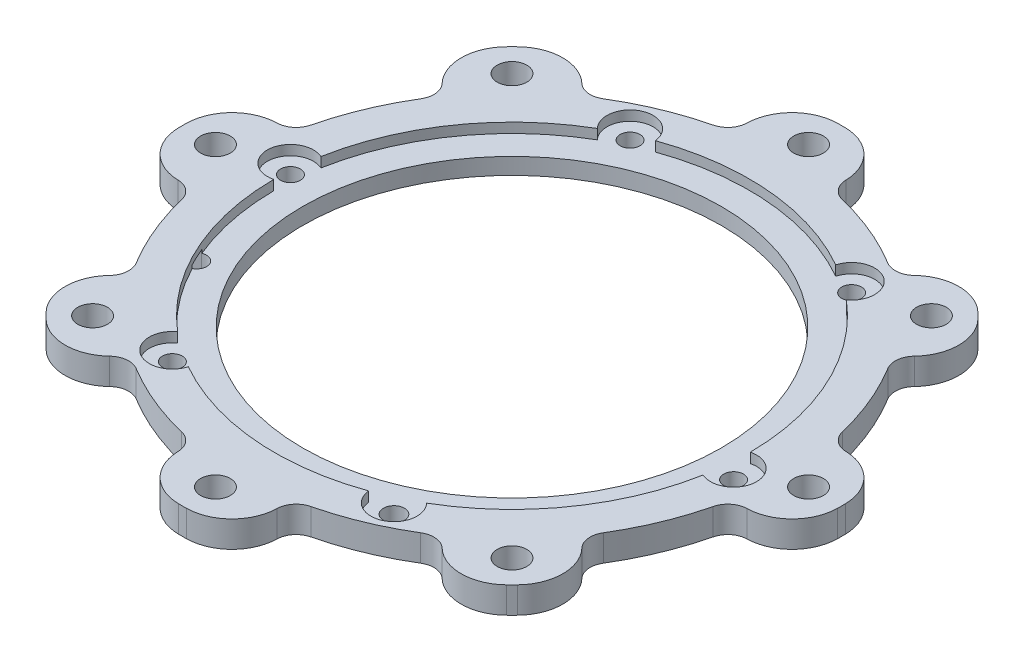
from build123d import *

# Parameters (mm, degrees)
SKETCH1_R           = 50
SKETCH1_R_2         = 30
BOSS_EXTRUDE1_DEPTH = 4
SKETCH2_R           = 39
SKETCH2_R_2         = 30
BOSS_EXTRUDE2_DEPTH = 1
SKETCH3_R           = 31.75
CUT_EXTRUDE1_DEPTH  = 1
SKETCH4_R           = 2.25
CUT_EXTRUDE2_DEPTH  = 10
CIRPATTERN1_COUNT   = 8
SKETCH5_R           = 31.75
CUT_EXTRUDE3_DEPTH  = 27
SKETCH6_R           = 3.5
CUT_EXTRUDE4_DEPTH  = 2.5
CIRPATTERN2_COUNT   = 6
SKETCH7_R           = 1.5
SKETCH7_R_2         = 1.597835056
CUT_EXTRUDE5_DEPTH  = 15
CUT_EXTRUDE6_DEPTH  = 13
CIRPATTERN3_COUNT   = 8
FILLET1_R           = 3
SKETCH9_R           = 36
CUT_EXTRUDE7_DEPTH  = 2.5
FILLET2_R           = 7
CUT_EXTRUDE8_START  = -1
SKETCH10_R          = 50
CUT_EXTRUDE8_DEPTH  = 1
SKETCH12_R          = 1.5
CUT_EXTRUDE9_DEPTH  = 3
CUT_EXTRUDE10_REACH = 72.824


with BuildPart() as part:
    # Sketch1 → Boss-Extrude1 (new body)
    with BuildSketch(Plane(origin=(0, 0, 0), x_dir=(1, 0, 0), z_dir=(0, 1, 0))):
        with Locations(Location((0, 0, 0), (0, 0, 270))):
            Circle(SKETCH1_R)
        with Locations(Location((0, 0, 0), (0, 0, 270))):
            Circle(SKETCH1_R_2, mode=Mode.SUBTRACT)
    extrude(amount=BOSS_EXTRUDE1_DEPTH)

    # Sketch2 → Boss-Extrude2 (add)
    with BuildSketch(Plane(origin=(0, 4, 0), x_dir=(1, 0, 0), z_dir=(0, 1, 0))):
        with Locations(Location((0, 0, 0), (0, 0, 270))):
            Circle(SKETCH2_R)
        with Locations(Location((0, 0, 0), (0, 0, 270))):
            Circle(SKETCH2_R_2, mode=Mode.SUBTRACT)
    extrude(amount=BOSS_EXTRUDE2_DEPTH)

    # Sketch3 → Cut-Extrude1 (cut)
    with BuildSketch(Plane.XZ):
        with Locations(Location((0, 0, 0), (0, 0, 270))):
            Circle(SKETCH3_R)
    extrude(amount=-CUT_EXTRUDE1_DEPTH, mode=Mode.SUBTRACT)

    # Sketch4 → Cut-Extrude2 (cut)
    with BuildSketch(Plane.XZ):
        with Locations(Location((0, 45, 0), (0, 0, 270))):
            Circle(SKETCH4_R)
    cut_extrude2 = extrude(amount=-CUT_EXTRUDE2_DEPTH, mode=Mode.SUBTRACT)

    # CirPattern1: Cut-Extrude2 ×8 about axis
    cirpattern1_axis = Axis((0, 0, 0), (0, 1, 0))
    for i in range(1, CIRPATTERN1_COUNT):
        add(cut_extrude2.rotate(cirpattern1_axis, i * 360 / CIRPATTERN1_COUNT), mode=Mode.SUBTRACT)

    # Sketch5 → Cut-Extrude3 (cut)
    with BuildSketch(Plane.XZ):
        with Locations(Location((0, 0, 0), (0, 0, 270))):
            Circle(SKETCH5_R)
    extrude(amount=-CUT_EXTRUDE3_DEPTH, mode=Mode.SUBTRACT)

    # Sketch6 → Cut-Extrude4 (cut)
    with BuildSketch(Plane(origin=(0, 5, 0), x_dir=(1, 0, 0), z_dir=(0, 1, 0))):
        with Locations(Location((36.858075929, -3.237628574, 0), (0, 0, 270))):
            Circle(SKETCH6_R)
    cut_extrude4 = extrude(amount=-CUT_EXTRUDE4_DEPTH, mode=Mode.SUBTRACT)

    # CirPattern2: Cut-Extrude4 ×6 about axis
    cirpattern2_axis = Axis((0, 0, 0), (0, 1, 0))
    for i in range(1, CIRPATTERN2_COUNT):
        add(cut_extrude4.rotate(cirpattern2_axis, i * 360 / CIRPATTERN2_COUNT), mode=Mode.SUBTRACT)

    # Sketch7 → Cut-Extrude5 (cut)
    with BuildSketch(Plane(origin=(0, 5, 0), x_dir=(1, 0, 0), z_dir=(0, 1, 0))):
        with Locations(Location((-21.232906558, -30.301215802, 0), (0, 0, 270))):
            Circle(SKETCH7_R)
        with Locations(Location((15.625169371, -33.538844377, 0), (0, 0, 270))):
            Circle(SKETCH7_R_2)
        with Locations(Location((36.858075929, -3.237628574, 0), (0, 0, 270))):
            Circle(SKETCH7_R)
        with Locations(Location((21.232906558, 30.301215802, 0), (0, 0, 270))):
            Circle(SKETCH7_R)
        with Locations(Location((-15.625169371, 33.538844377, 0), (0, 0, 270))):
            Circle(SKETCH7_R)
        with Locations(Location((-36.858075929, 3.237628574, 0), (0, 0, 270))):
            Circle(SKETCH7_R)
    extrude(amount=-CUT_EXTRUDE5_DEPTH, mode=Mode.SUBTRACT)

    # Sketch8 → Cut-Extrude6 (cut)
    with BuildSketch(Plane.XZ):
        with BuildLine():
            Line((7.5, -40.816663264), (7.5, -49.434299833))
            ThreePointArc((7.5, -49.434299833), (19.134171618, -46.193976626), (29.652027776, -40.258629494))
            Line((29.652027776, -40.258629494), (23.55843852, -34.165040238))
            ThreePointArc((23.55843852, -34.165040238), (15.881362443, -38.341000599), (7.5, -40.816663264))
        make_face()
    cut_extrude6 = extrude(amount=-CUT_EXTRUDE6_DEPTH, mode=Mode.SUBTRACT)

    # CirPattern3: Cut-Extrude6 ×8 about axis
    cirpattern3_axis = Axis((0, 0, 0), (0, 1, 0))
    for i in range(1, CIRPATTERN3_COUNT):
        add(cut_extrude6.rotate(cirpattern3_axis, i * 360 / CIRPATTERN3_COUNT), mode=Mode.SUBTRACT)

    # Fillet1
    fillet1_edges = [part.edges().sort_by_distance(p)[0] for p in [
        (7.5, 2, -40.816663264),
        (23.55843852, 2, -34.165040238),
        (34.165040238, 2, -23.55843852),
        (40.816663264, 2, -7.5),
        (40.816663264, 2, 7.5),
        (34.165040238, 2, 23.55843852),
        (23.55843852, 2, 34.165040238),
        (7.5, 2, 40.816663264),
        (-7.5, 2, 40.816663264),
        (-23.55843852, 2, 34.165040238),
        (-34.165040238, 2, 23.55843852),
        (-40.816663264, 2, 7.5),
        (-40.816663264, 2, -7.5),
        (-34.165040238, 2, -23.55843852),
        (-23.55843852, 2, -34.165040238),
        (-7.5, 2, -40.816663264),
    ]]
    fillet(fillet1_edges, radius=FILLET1_R)

    # Sketch9 → Cut-Extrude7 (cut)
    with BuildSketch(Plane(origin=(0, 5, 0), x_dir=(1, 0, 0), z_dir=(0, 1, 0))):
        Circle(SKETCH9_R)
    extrude(amount=-CUT_EXTRUDE7_DEPTH, mode=Mode.SUBTRACT)

    # Fillet2
    fillet2_edges = [part.edges().sort_by_distance(p)[0] for p in [
        (40.258629494, 2, -29.652027776),
        (29.652027776, 2, -40.258629494),
        (7.5, 2, -49.434299833),
        (-7.5, 2, -49.434299833),
        (-29.652027776, 2, -40.258629494),
        (-40.258629494, 2, -29.652027776),
        (-49.434299833, 2, -7.5),
        (-49.434299833, 2, 7.5),
        (-40.258629494, 2, 29.652027776),
        (-29.652027776, 2, 40.258629494),
        (-7.5, 2, 49.434299833),
        (7.5, 2, 49.434299833),
        (29.652027776, 2, 40.258629494),
        (40.258629494, 2, 29.652027776),
        (49.434299833, 2, 7.5),
        (49.434299833, 2, -7.5),
    ]]
    fillet(fillet2_edges, radius=FILLET2_R)

    # Sketch10 → Cut-Extrude8 (cut)
    with BuildSketch(Plane(origin=(0, 5, 0), x_dir=(1, 0, 0), z_dir=(0, 1, 0)).offset(CUT_EXTRUDE8_START)):
        Circle(SKETCH10_R)
    extrude(amount=CUT_EXTRUDE8_DEPTH, mode=Mode.SUBTRACT)

    # Sketch12 → Cut-Extrude9 (cut)
    with BuildSketch(Plane.XZ):
        with Locations(Location((-33.538844377, 15.625169371, 0), (0, 0, 270))):
            Circle(SKETCH12_R)
        with Locations(Location((33.538844377, -15.625169371, 0), (0, 0, 270))):
            Circle(SKETCH12_R)
    extrude(amount=-CUT_EXTRUDE9_DEPTH, mode=Mode.SUBTRACT)

    # Cut-Extrude10: up to this face of the body (flat: up to its plane)
    cut_extrude10_end = Plane(part.part.faces().sort_by_distance((-33.670920616, 3, 15.686701414))[0])
    # Sketch13 → Cut-Extrude10 (cut, up to the picked face)
    with BuildSketch(Plane.XZ, mode=Mode.PRIVATE) as cut_extrude10_sk1:
        with BuildLine():
            Line((-33.265841936, 13.843184616), (-35.078752442, 14.687788366))
            ThreePointArc((-35.078752442, 14.687788366), (-35.80498251, 16.680924059), (-33.811846818, 17.407154126))
            Line((-33.811846818, 17.407154126), (-31.998936311, 16.562550377))
            ThreePointArc((-31.998936311, 16.562550377), (-31.272706243, 14.569414684), (-33.265841936, 13.843184616))
        make_face()
    cut_extrude10_tool1 = split(extrude(cut_extrude10_sk1.sketch, amount=-CUT_EXTRUDE10_REACH, mode=Mode.PRIVATE), bisect_by=cut_extrude10_end, keep=Keep.BOTH, mode=Mode.PRIVATE)
    add(cut_extrude10_tool1.solids().sort_by(Axis((-33.538844, 0, 15.625169), (0, 1, 0)))[0], mode=Mode.SUBTRACT)


solid = part.part
